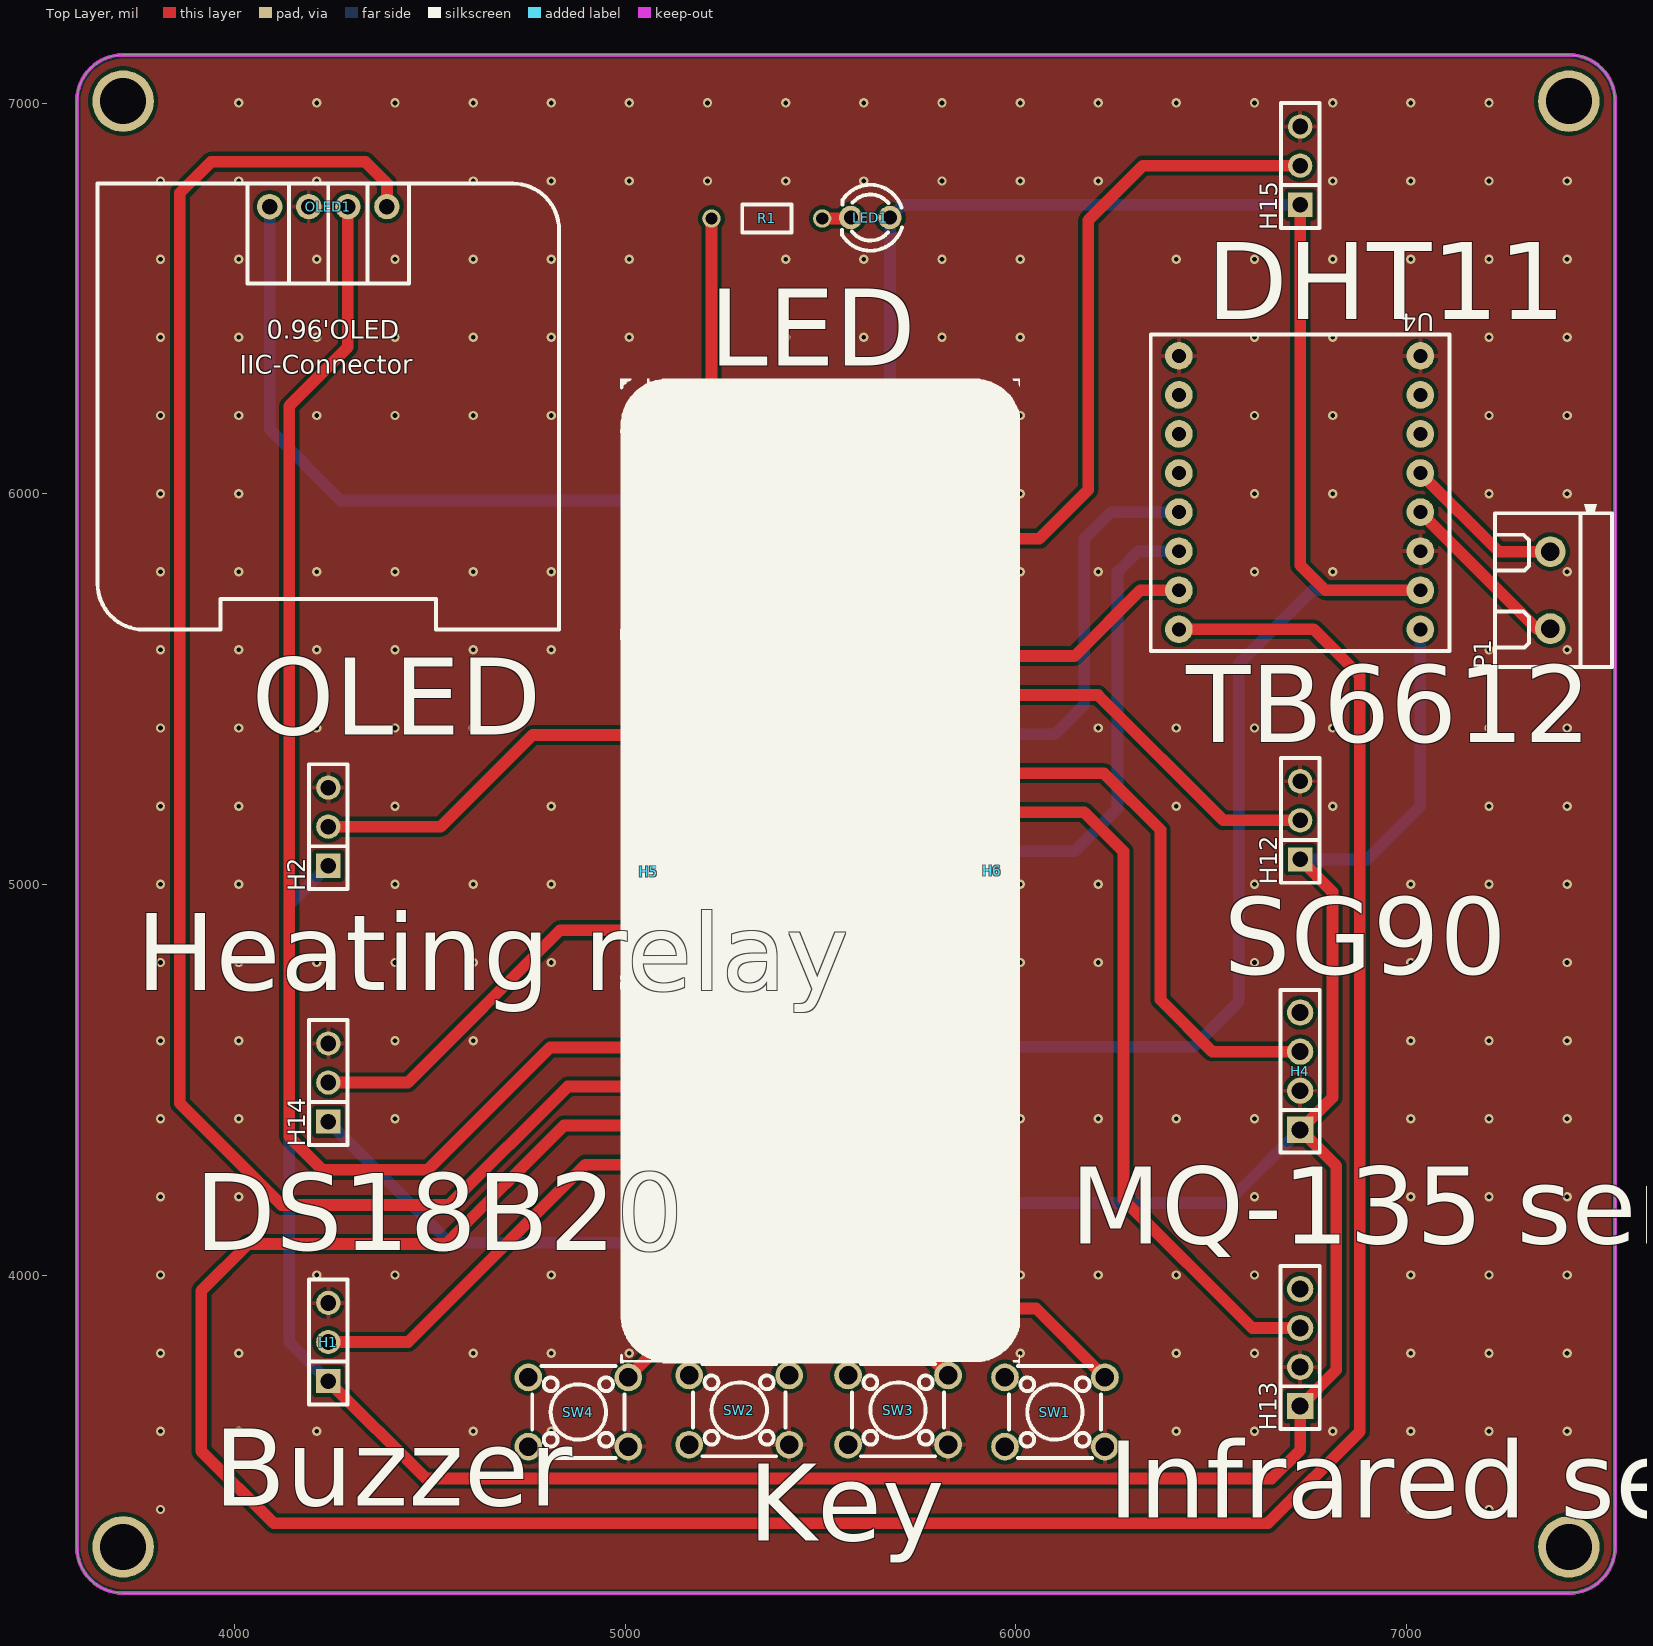
[diagram p0: Top Layer view]
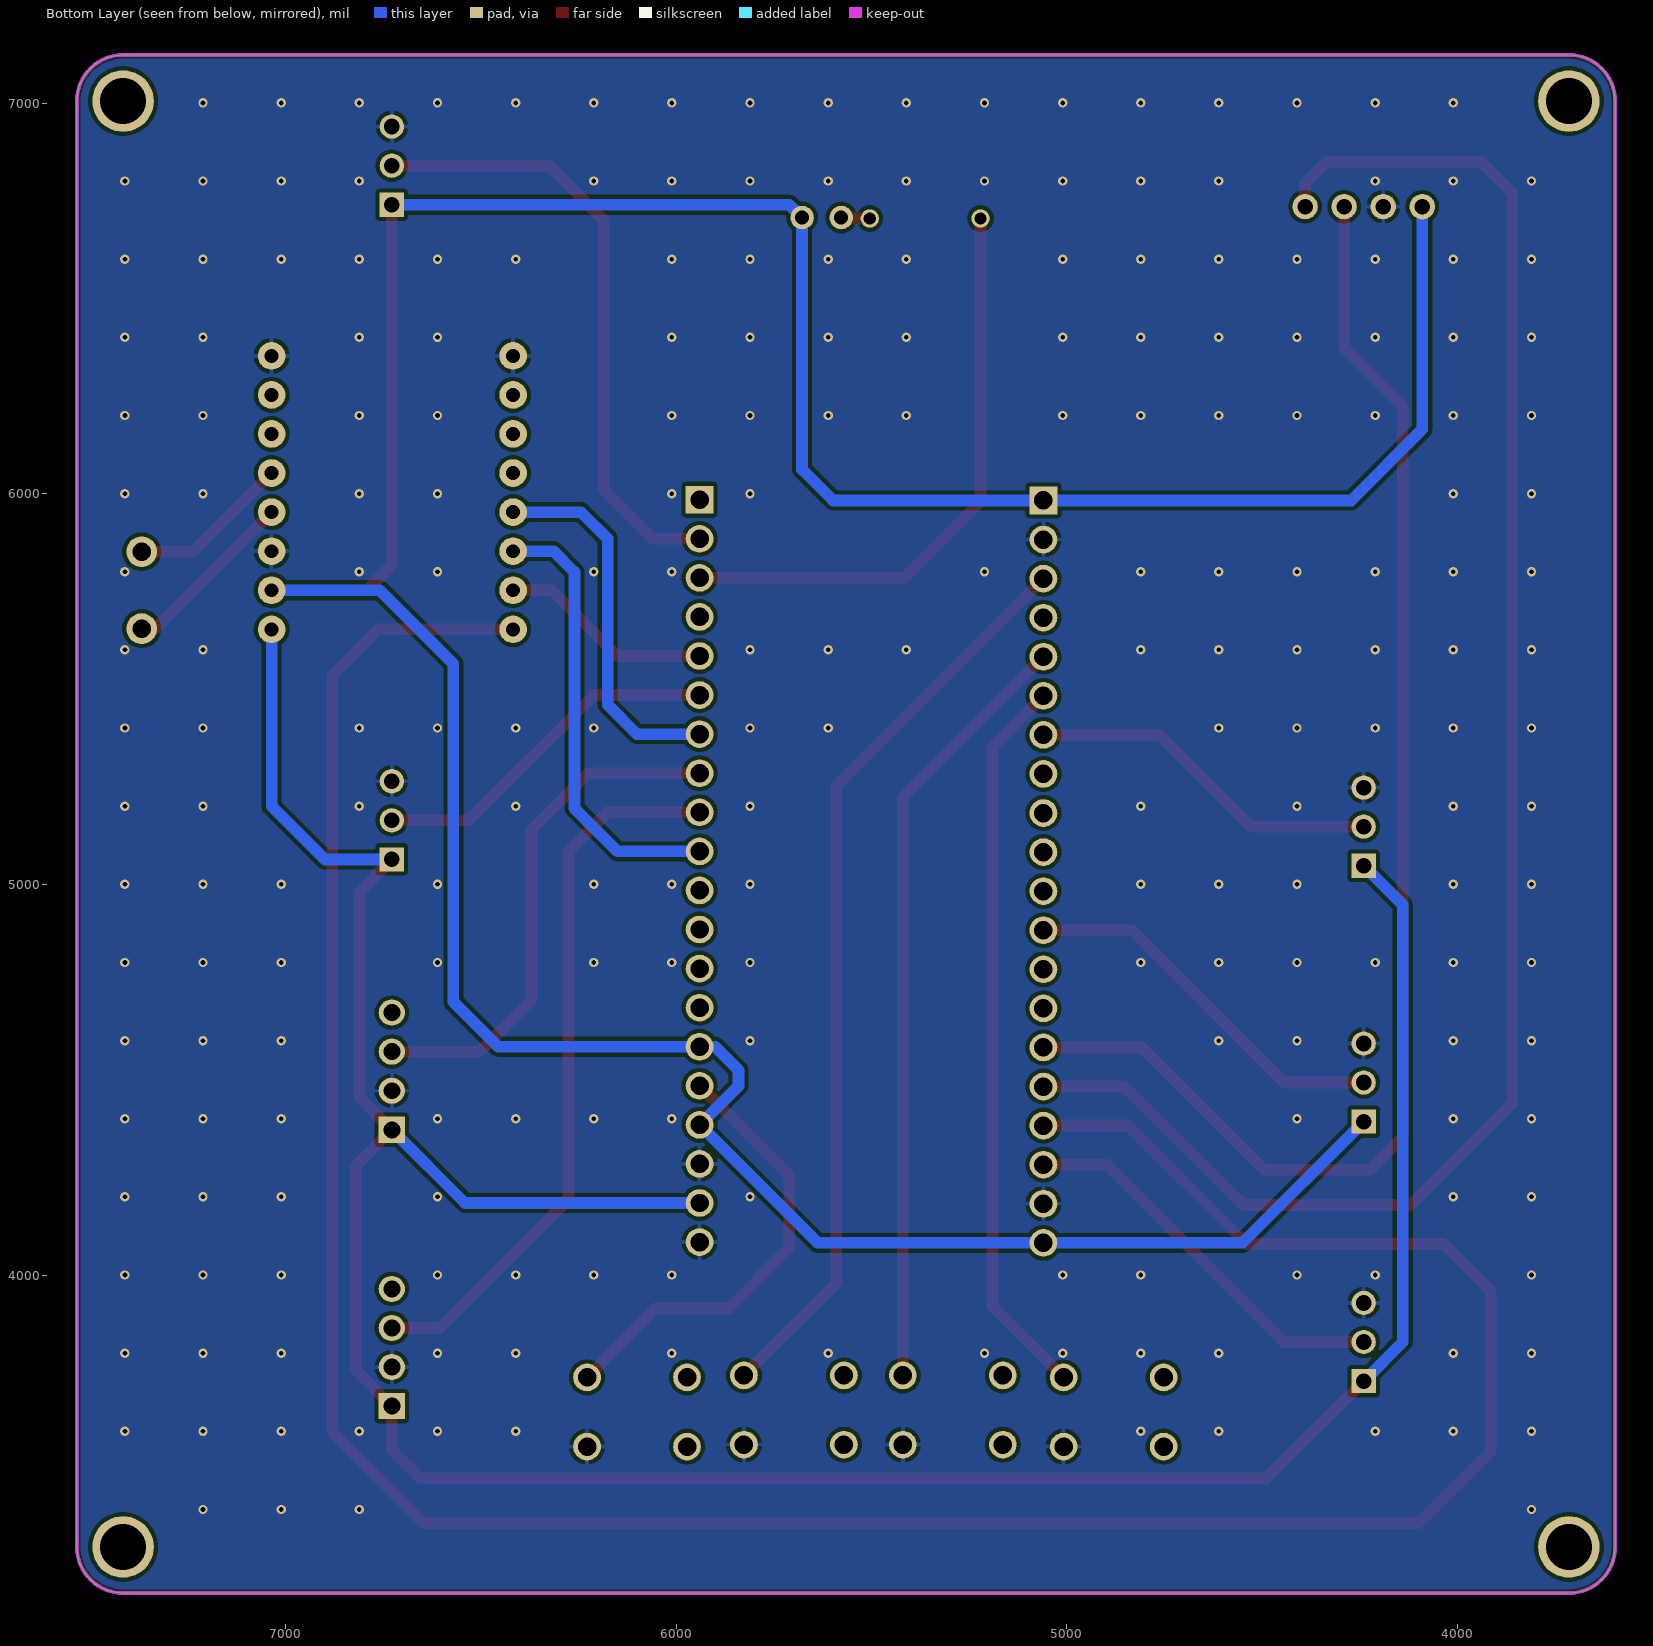
[diagram p1: Bottom Layer view, seen from below]
# Altium PCB MISC49946.pcbdoc
Units mil, origin at the board's own origin, x right, y up, seen from the top; angles counter-clockwise.
Board outline 3937.01 x 3937.01 mil, 2 copper layers (Top Layer, Bottom Layer), stack 62.206 mil thick; 18 components, 37 nets, 109 pads, 223 vias.

## Layer stack, top to bottom
Top Solder Mask Layer: solder mask 0.394, Dk 3.3
Top Layer: signal copper 1.379
Dielectric1: surface 59.449, FR4, Dk 4.5
Bottom Layer: signal copper 1.378
Bottom Solder Mask Layer: solder mask 0.394, Dk 3.3

## Board outline
3714.61,7123.5 ccw(c3714.61,7005.39) 3596.5,7005.39 3596.5,3304.61 ccw(c3714.61,3304.61) 3714.61,3186.5 7415.39,3186.5 ccw(c7415.39,3304.61) 7533.5,3304.61 7533.5,7005.39 ccw(c7415.39,7005.39) 7415.39,7123.5 3714.61,7123.5

## Design rules (kind name [scope] priority, off if disabled: settings)
BoardOutlineClearance copperThickness2oz_1 [All] p2 off: genericclearance=7.99 ignorepadtopadclearanceinfootprint=FALSE except(0: Arc-SplitContinuation Track-SplitContinuation SMDPad-SplitContinuation THPad-SplitContinuation Via-SplitContinuation Fill-SplitContinuation Region-SplitContinuation Poly-SplitContinuation Text-SplitContinuation Hole-SplitContinuation; 5.98: Arc-CutoutEdge Track-CutoutEdge SMDPad-CutoutEdge THPad-CutoutEdge Via-CutoutEdge Text-CutoutEdge; 6.9: Hole-OutlineEdge Hole-CutoutEdge; 10: Poly-OutlineEdge Poly-CutoutEdge; 11.81: Arc-OutlineEdge Track-OutlineEdge SMDPad-OutlineEdge THPad-OutlineEdge Via-OutlineEdge Fill-OutlineEdge Region-OutlineEdge Text-OutlineEdge Fill-CutoutEdge Region-CutoutEdge)
BoardOutlineClearance Plane_innerPlane_1 [All] p4 off: genericclearance=4.02 ignorepadtopadclearanceinfootprint=FALSE except(0: Arc-SplitContinuation Track-SplitContinuation SMDPad-SplitContinuation THPad-SplitContinuation Via-SplitContinuation Fill-SplitContinuation Region-SplitContinuation Poly-SplitContinuation Text-SplitContinuation Hole-SplitContinuation; 5.98: Arc-CutoutEdge Track-CutoutEdge SMDPad-CutoutEdge THPad-CutoutEdge Via-CutoutEdge Text-CutoutEdge; 6.9: Hole-OutlineEdge Hole-CutoutEdge; 10: Poly-OutlineEdge Poly-CutoutEdge; 11.81: Arc-OutlineEdge Track-OutlineEdge SMDPad-OutlineEdge THPad-OutlineEdge Via-OutlineEdge Fill-OutlineEdge Region-OutlineEdge Text-OutlineEdge Fill-CutoutEdge Region-CutoutEdge)
BoardOutlineClearance Copper_copperRegion_1 [All] p6 off: genericclearance=4.02 ignorepadtopadclearanceinfootprint=FALSE except(0: Arc-SplitContinuation Track-SplitContinuation SMDPad-SplitContinuation THPad-SplitContinuation Via-SplitContinuation Fill-SplitContinuation Region-SplitContinuation Poly-SplitContinuation Text-SplitContinuation Hole-SplitContinuation; 5.98: Arc-CutoutEdge Track-CutoutEdge SMDPad-CutoutEdge THPad-CutoutEdge Via-CutoutEdge Text-CutoutEdge; 6.9: Hole-OutlineEdge Hole-CutoutEdge; 10: Poly-OutlineEdge Poly-CutoutEdge; 11.81: Arc-OutlineEdge Track-OutlineEdge SMDPad-OutlineEdge THPad-OutlineEdge Via-OutlineEdge Fill-OutlineEdge Region-OutlineEdge Text-OutlineEdge Fill-CutoutEdge Region-CutoutEdge)
BoardOutlineClearance Copper_copperRegion_copperThickness1oz_1 [All] p8 off: genericclearance=4.02 ignorepadtopadclearanceinfootprint=FALSE except(0: Arc-SplitContinuation Track-SplitContinuation SMDPad-SplitContinuation THPad-SplitContinuation Via-SplitContinuation Fill-SplitContinuation Region-SplitContinuation Poly-SplitContinuation Text-SplitContinuation Hole-SplitContinuation; 5.98: Arc-CutoutEdge Track-CutoutEdge SMDPad-CutoutEdge THPad-CutoutEdge Via-CutoutEdge Text-CutoutEdge; 6.9: Hole-OutlineEdge Hole-CutoutEdge; 10: Poly-OutlineEdge Poly-CutoutEdge; 11.81: Arc-OutlineEdge Track-OutlineEdge SMDPad-OutlineEdge THPad-OutlineEdge Via-OutlineEdge Fill-OutlineEdge Region-OutlineEdge Text-OutlineEdge Fill-CutoutEdge Region-CutoutEdge)
BoardOutlineClearance Copper_copperRegion_Copper_copperRegion_1 [All] p10 off: genericclearance=4.02 ignorepadtopadclearanceinfootprint=FALSE except(0: Arc-SplitContinuation Track-SplitContinuation SMDPad-SplitContinuation THPad-SplitContinuation Via-SplitContinuation Fill-SplitContinuation Region-SplitContinuation Poly-SplitContinuation Text-SplitContinuation Hole-SplitContinuation; 5.98: Arc-CutoutEdge Track-CutoutEdge SMDPad-CutoutEdge THPad-CutoutEdge Via-CutoutEdge Text-CutoutEdge; 6.9: Hole-OutlineEdge Hole-CutoutEdge; 10: Poly-OutlineEdge Poly-CutoutEdge; 11.81: Arc-OutlineEdge Track-OutlineEdge SMDPad-OutlineEdge THPad-OutlineEdge Via-OutlineEdge Fill-OutlineEdge Region-OutlineEdge Text-OutlineEdge Fill-CutoutEdge Region-CutoutEdge)
BoardOutlineClearance copperThickness1oz_1 [All] p12: genericclearance=4.02 ignorepadtopadclearanceinfootprint=FALSE except(0: Arc-SplitContinuation Track-SplitContinuation SMDPad-SplitContinuation THPad-SplitContinuation Via-SplitContinuation Fill-SplitContinuation Region-SplitContinuation Poly-SplitContinuation Text-SplitContinuation Hole-SplitContinuation; 5.98: Arc-CutoutEdge Track-CutoutEdge SMDPad-CutoutEdge THPad-CutoutEdge Via-CutoutEdge Text-CutoutEdge; 6.9: Hole-OutlineEdge Hole-CutoutEdge; 10: Poly-OutlineEdge Poly-CutoutEdge; 11.81: Arc-OutlineEdge Track-OutlineEdge SMDPad-OutlineEdge THPad-OutlineEdge Via-OutlineEdge Fill-OutlineEdge Region-OutlineEdge Text-OutlineEdge Fill-CutoutEdge Region-CutoutEdge)
Clearance copperThickness2oz [All] p1 off: gap=7.99 ignorepadtopadclearanceinfootprint=FALSE except(5.98: SMDPad-Track SMDPad-SMDPad THPad-Track SMDPad-THPad THPad-THPad Track-Via SMDPad-Via THPad-Via Via-Via Fill-SMDPad Region-SMDPad Fill-THPad Region-THPad Fill-Via Region-Via Fill-Fill Fill-Region Region-Region Arc-Track Arc-SMDPad Arc-THPad Arc-Via Fill-Arc Region-Arc Arc-Arc Text-Track SMDPad-Text Text-THPad Text-Via Fill-Text Region-Text Arc-Text Text-Text; 6.9: Hole-Track Hole-SMDPad Hole-THPad Hole-Via Fill-Hole Region-Hole Hole-Arc Hole-Text; 10: Poly-Track Poly-SMDPad Poly-THPad Poly-Via Poly-Fill Poly-Region Poly-Poly Poly-Arc Poly-Text Poly-Hole; 11.81: Fill-Track Region-Track)
Clearance Plane_innerPlane [All] p3 off: gap=4.02 ignorepadtopadclearanceinfootprint=FALSE except(5.98: SMDPad-Track SMDPad-SMDPad THPad-Track SMDPad-THPad THPad-THPad Track-Via SMDPad-Via THPad-Via Via-Via Fill-SMDPad Region-SMDPad Fill-THPad Region-THPad Fill-Via Region-Via Fill-Fill Fill-Region Region-Region Arc-Track Arc-SMDPad Arc-THPad Arc-Via Fill-Arc Region-Arc Arc-Arc Text-Track SMDPad-Text Text-THPad Text-Via Fill-Text Region-Text Arc-Text Text-Text; 6.9: Hole-Track Hole-SMDPad Hole-THPad Hole-Via Fill-Hole Region-Hole Hole-Arc Hole-Text; 10: Poly-Track Poly-SMDPad Poly-THPad Poly-Via Poly-Fill Poly-Region Poly-Poly Poly-Arc Poly-Text Poly-Hole; 11.81: Fill-Track Region-Track)
Clearance Copper_copperRegion [All] p5 off: gap=4.02 ignorepadtopadclearanceinfootprint=FALSE except(5.98: SMDPad-Track SMDPad-SMDPad THPad-Track SMDPad-THPad THPad-THPad Track-Via SMDPad-Via THPad-Via Via-Via Fill-SMDPad Region-SMDPad Fill-THPad Region-THPad Fill-Via Region-Via Fill-Fill Fill-Region Region-Region Arc-Track Arc-SMDPad Arc-THPad Arc-Via Fill-Arc Region-Arc Arc-Arc Text-Track SMDPad-Text Text-THPad Text-Via Fill-Text Region-Text Arc-Text Text-Text; 6.9: Hole-Track Hole-SMDPad Hole-THPad Hole-Via Fill-Hole Region-Hole Hole-Arc Hole-Text; 10: Poly-Track Poly-SMDPad Poly-THPad Poly-Via Poly-Fill Poly-Region Poly-Poly Poly-Arc Poly-Text Poly-Hole; 11.81: Fill-Track Region-Track)
Clearance Copper_copperRegion_copperThickness1oz [All] p7 off: gap=4.02 ignorepadtopadclearanceinfootprint=FALSE except(5.98: SMDPad-Track SMDPad-SMDPad THPad-Track SMDPad-THPad THPad-THPad Track-Via SMDPad-Via THPad-Via Via-Via Fill-SMDPad Region-SMDPad Fill-THPad Region-THPad Fill-Via Region-Via Fill-Fill Fill-Region Region-Region Arc-Track Arc-SMDPad Arc-THPad Arc-Via Fill-Arc Region-Arc Arc-Arc Text-Track SMDPad-Text Text-THPad Text-Via Fill-Text Region-Text Arc-Text Text-Text; 6.9: Hole-Track Hole-SMDPad Hole-THPad Hole-Via Fill-Hole Region-Hole Hole-Arc Hole-Text; 10: Poly-Track Poly-SMDPad Poly-THPad Poly-Via Poly-Fill Poly-Region Poly-Poly Poly-Arc Poly-Text Poly-Hole; 11.81: Fill-Track Region-Track)
Clearance Copper_copperRegion_Copper_copperRegion [All] p9 off: gap=4.02 ignorepadtopadclearanceinfootprint=FALSE except(5.98: SMDPad-Track SMDPad-SMDPad THPad-Track SMDPad-THPad THPad-THPad Track-Via SMDPad-Via THPad-Via Via-Via Fill-SMDPad Region-SMDPad Fill-THPad Region-THPad Fill-Via Region-Via Fill-Fill Fill-Region Region-Region Arc-Track Arc-SMDPad Arc-THPad Arc-Via Fill-Arc Region-Arc Arc-Arc Text-Track SMDPad-Text Text-THPad Text-Via Fill-Text Region-Text Arc-Text Text-Text; 6.9: Hole-Track Hole-SMDPad Hole-THPad Hole-Via Fill-Hole Region-Hole Hole-Arc Hole-Text; 10: Poly-Track Poly-SMDPad Poly-THPad Poly-Via Poly-Fill Poly-Region Poly-Poly Poly-Arc Poly-Text Poly-Hole; 11.81: Fill-Track Region-Track)
Clearance copperThickness1oz [All] p11: gap=4.02 ignorepadtopadclearanceinfootprint=FALSE except(5.98: SMDPad-Track SMDPad-SMDPad THPad-Track SMDPad-THPad THPad-THPad Track-Via SMDPad-Via THPad-Via Via-Via Fill-SMDPad Region-SMDPad Fill-THPad Region-THPad Fill-Via Region-Via Fill-Fill Fill-Region Region-Region Arc-Track Arc-SMDPad Arc-THPad Arc-Via Fill-Arc Region-Arc Arc-Arc Text-Track SMDPad-Text Text-THPad Text-Via Fill-Text Region-Text Arc-Text Text-Text; 6.9: Hole-Track Hole-SMDPad Hole-THPad Hole-Via Fill-Hole Region-Hole Hole-Arc Hole-Text; 10: Poly-Track Poly-SMDPad Poly-THPad Poly-Via Poly-Fill Poly-Region Poly-Poly Poly-Arc Poly-Text Poly-Hole; 11.81: Fill-Track Region-Track)
DiffPairsRouting differentialPair [All] p1: maxlimit=6 minlimit=6 mostfreqgap=6 toplayer_minwidth=5 toplayer_prefwidth=10 toplayer_maxwidth=100 toplayer_mingap=6 toplayer_prefgap=6 toplayer_maxgap=6 bottomlayer_minwidth=5 bottomlayer_prefwidth=10 bottomlayer_maxwidth=100 bottomlayer_mingap=6 bottomlayer_prefgap=6 bottomlayer_maxgap=6 maxuncoupledlength=10
HoleToHoleClearance otherClearance [All] p1: gap=11.81 allowstackedmicrovias=TRUE
Length netLength [All] p1: minlimit=0 maxlimit=0
PasteMaskExpansion pasteMaskExpansion [All] p1: expansion=0
PlaneConnect innerPlane [All] p1: planeconnectstyle=Relief reliefexpansion=20 reliefentries=4 reliefconductorwidth=10 reliefairgap=10
PolygonConnect copperRegion_copperThickness1oz [All] p1 off: connectstyle=Relief reliefconductorwidth=10 reliefentries=4 polygonreliefangle="90 Angle" airgapwidth=10 via.connectstyle=Relief via.reliefconductorwidth=10 via.reliefentries=4 via.polygonreliefangle="90 Angle" via.airgapwidth=10
PolygonConnect copperRegion_Copper_copperRegion [All] p2 off: connectstyle=Relief reliefconductorwidth=10 reliefentries=4 polygonreliefangle="90 Angle" airgapwidth=10 via.connectstyle=Relief via.reliefconductorwidth=10 via.reliefentries=4 via.polygonreliefangle="90 Angle" via.airgapwidth=10
PolygonConnect copperRegion [All] p3: connectstyle=Relief reliefconductorwidth=10 reliefentries=4 polygonreliefangle="90 Angle" airgapwidth=10 via.connectstyle=Relief via.reliefconductorwidth=10 via.reliefentries=4 via.polygonreliefangle="90 Angle" via.airgapwidth=10
RoutingVias viaSize [All] p1: holewidth=12.01 width=24.02 viastyle="Through Hole" minholewidth=11.81 minwidth=19.68 maxholewidth=248.03 maxwidth=393.7
SolderMaskExpansion solderMaskExpansion [IsVia] p1: expansion=-1000 istentingtop=TRUE
SolderMaskExpansion solderMaskExpansion [All] p2: expansion=2 istentingtop=FALSE
Width copperThickness2oz_2 [All] p1 off: maxlimit=100 minlimit=8 preferedwidth=10
Width copperThickness1oz_2 [All] p2: maxlimit=100 minlimit=5 preferedwidth=10

## Components (designator, comment, footprint, x,y, rotation, side; value= is the part's Value field where it differs from the comment)
H1 "" HDR-TH_3P-P2.54-V-F 4240,3829.14 r90 top
H2 "" HDR-TH_3P-P2.54-V-F 4240,5148.1 r90 top
H4 "" HDR-TH_4P-P2.54-V-F 6727.5,4522.29 r90 top
H5 "" HDR-TH_20P-P2.54-V-F 5059.74,5033.05 r270 top
H6 "" HDR-TH_20P-P2.54-V-F 5939.74,5034.94 r270 top
H12 "" HDR-TH_3P-P2.54-V-F 6727.5,5164.4 r90 top
H13 "" HDR-TH_4P-P2.54-V-F 6727.5,3815.05 r90 top
H14 "" HDR-TH_3P-P2.54-V-F 4240,4493.24 r90 top
H15 "" HDR-TH_3P-P2.54-V-F 6727.5,6840 r90 top
LED1 "" LED_TH-3mm 5627.35,6707.23 r180 top
OLED1 "" 0.96OLED_4P 4240,6735 r0 top
P1 "KF301-2P terminal block" CONN-TH_XY301V-A-5.0-2P 7367.76,5753.51 r90 top
R1 "220Ω" Res_1/8W 5362.36,6707.23 r180 top
SW1 "" SW-TH_4P-L6.0-W6.0-P4.50-LS6.5 6099.85,3650 r180 top
SW2 "" SW-TH_4P-L6.0-W6.0-P4.50-LS6.5 5291.62,3655 r180 top
SW3 "" SW-TH_4P-L6.0-W6.0-P4.50-LS6.5 5698.23,3655 r180 top
SW4 "" SW-TH_4P-L6.0-W6.0-P4.50-LS6.5 4880,3650 r180 top
U4 "" tb6612 7035,5653.24 r180 top

## Footprints (in the part's own frame and the unit in brackets; to place one, negate y for a bottom-side part, rotate by r counter-clockwise, add the part's x,y. Pads: shape width x height; smd on the part's side, far side on the other; paste and mask are expansions set on the pad)
0.96OLED_4P [mm]
  round 1.65 hole 1 copper offset 0,0: 1(-3.81,-0.001) 2(-1.27,0.002) 3(1.27,0.002) 4(3.81,0.002)
  silkscreen extent -15,-27.5 15,1.5
CONN-TH_XY301V-A-5.0-2P [mm]
  round 2 hole 1.2: 1(-2.5,0) 2(2.5,0)
  silkscreen extent -5,-4 5.6,3.6
HDR-TH_3P-P2.54-V-F [mil]
  rect 62x62 hole 40.16: 1(-100,0)
  round 62 hole 40.16: 2(0,0) 3(100,0)
  silkscreen extent -160,-49 160,49
HDR-TH_4P-P2.54-V-F [mm]
  rect 1.7x1.7 hole 1.1: 1(-3.81,0)
  round 1.7 hole 1.1: 2(-1.27,0) 3(1.27,0) 4(3.81,0)
  silkscreen extent -5.29,-1.27 5.29,1.27
HDR-TH_20P-P2.54-V-F [mm]
  rect 1.8x1.8 hole 1.2: 1(-24.13,0)
  round 1.8 hole 1.2: 2(-21.59,0) 3(-19.05,0) 4(-16.51,0) 5(-13.97,0) 6(-11.43,0) 7(-8.89,0) 8(-6.35,0) 9(-3.81,0) 10(-1.27,0) 11(1.27,0) 12(3.81,0) 13(6.35,0) 14(8.89,0) 15(11.43,0) 16(13.97,0) 17(16.51,0) 18(19.05,0) 19(21.59,0) 20(24.13,0)
  silkscreen extent -25.65,-1.25 25.65,1.25
LED_TH-3mm [mil]
  round 60 hole 36 paste+0 mask+2: 1(-50,0) 2(50,0)
  silkscreen extent -81,-84 72,85
Res_1/8W [mil]
  round 47.2 hole 31.5 paste+0 mask+2: 1(-141.7,2.48) 2(141.7,2.48)
  silkscreen extent -63,-33 63,38
SW-TH_4P-L6.0-W6.0-P4.50-LS6.5 [mm]
  round 1.8 hole 1.2: 1(-3.25,2.25) 2(3.25,2.25) 3(-3.25,-2.25) 4(3.25,-2.25)
  silkscreen extent -3,-3 3,3
tb6612 [mm]
  round 1.8 hole 0.9: 1(0,0) 2(0,-2.54) 3(0,-5.08) 4(0,-7.62) 5(0,-10.16) 6(0,-12.7) 7(0,-15.24) 8(0,-17.78) 9(15.697,-17.78) 10(15.697,-15.24) 11(15.697,-12.7) 12(15.697,-10.16) 13(15.697,-7.62) 14(15.697,-5.08) 15(15.697,-2.54) 16(15.697,0)
  silkscreen extent -1.91,-19.18 17.53,1.4

## Free pads (board coordinates)
  round 157.48 hole 118.11: 1(3714.61,7005.39) 1(3714.61,3304.61) 1(7415.39,7005.39) 1(7415.39,3304.61)

## Via types
v1: diameter 24.02, hole 12, Top Layer to Bottom Layer, 223 vias

## Nets (pads, with @x,y where several pads share a name; then routed paths per layer and width w, separated by ;. In a path a pad name is that pad's centre, name@x,y a point inside that pad or via, vN(x,y) a via of type N, cw(c..) or ccw(c..) an arc to the next point about the centre after c; other vN are vias at no path point)
$1N17195: LED1.2 R1.1 | length 74.3
  Top Layer w30: R1.1 5574.87,6704.75 LED1.2
$1N17231: P1.1 U4.4 | length 456.3
  Top Layer w30: U4.4 7333.15,5655.09 P1.1
$1N17232: P1.2 U4.5 | length 416.1
  Top Layer w30: U4.5 7236.3,5851.94 P1.2
+5V: H1.1 H2.1 H4.1 H6.19 H12.1 H13.1 U4.1 | length 7361.7
  Top Layer w30: H1.1 4489.14,3480 6655,3480 6727.5,3552.5 H13.1 6820,3757.55 6820,4279.79 H4.1 6810,4454.79 6810,4981.9 H12.1
  Bottom Layer w30: H1.1 4140,3829.14 4140,4948.1 H2.1 ; H6.19 6540.15,4184.94 H4.1 ; H12.1 6899.4,5064.4 7035,5200 U4.1
A0: H6.14
A1: H6.13
A2: H6.12
A3: H6.11
A4: H6.10 U4.14 | length 1149.9
  Bottom Layer w30: H6.10 6149.94,5084.94 6260,5195 6260,5800 6313.24,5853.24 U4.14
A5: H6.9 H13.3 | length 1855.8
  Top Layer w30: H6.9 6175.06,5184.94 6275,5085 6275,4195 6604.95,3865.05 H13.3
A6: H4.3 H6.8 | length 1337.8
  Top Layer w30: H6.8 6225.06,5284.94 6370,5140 6370,4705 6502.71,4572.29 H4.3
A7: H6.7 U4.13 | length 961.6
  Bottom Layer w30: H6.7 6099.94,5384.94 6175,5460 6175,5885 6243.24,5953.24 U4.13
A8: H2.2 H5.7 | length 917.1
  Top Layer w30: H2.2 4528.1,5148.1 4763.05,5383.05 H5.7
A9: H5.5 SW2.3 | length 1988.5
  Top Layer w30: H5.5 5419.57,5223.22 SW2.3
A10: H5.6 SW4.3 | length 1873.8
  Top Layer w30: SW4.3 5190,3920.63 5190,5352.79 H5.6
A11: H5.3 SW3.3 | length 2356.9
  Top Layer w30: H5.3 5590,5252.79 5590,3979.76 SW3.3
A12: H5.4
A15: H5.11
B0: H6.6 H12.2 | length 920.5
  Top Layer w30: H6.6 6210.06,5484.94 6530.6,5164.4 H12.2
B1: H6.5 U4.15 | length 547
  Top Layer w30: H6.5 6149.94,5584.94 6318.24,5753.24 U4.15
B3: H5.12 H14.2 | length 981.2
  Top Layer w30: H14.2 4443.24,4493.24 4833.05,4883.05 H5.12
B4: H5.13
B5: H5.14
B6: H5.15 OLED1.3 | length 3526.8
  Top Layer w30: OLED1.3@4290,6735.05 4290,6375 4140,6225 4140,4355 4225,4270 4495,4270 4808.05,4583.05 H5.15
B7: H5.16 OLED1.4 | length 4408.8
  Top Layer w30: OLED1.4@4390,6735.05 4390,6795 4335,6850 3940,6850 3860,6770 3860,4440 4120,4180 4550,4180 4853.05,4483.05 H5.16
B8: H5.17 U4.16 | length 7315.9
  Top Layer w30: H5.17 4843.05,4383.05 4540,4080 4035,4080 3915,3960 3915,3550 4100,3365 6645,3365 6880,3600 6880,5535 6761.76,5653.24 U4.16
B9: H1.2 H5.18 | length 1007.8
  Top Layer w30: H1.2 4444.14,3829.14 4898.05,4283.05 H5.18
B10: H6.4
B11: H6.3 R1.2 | length 1525
  Top Layer w30: R1.2 5220.66,5979.34 5415.06,5784.94 H6.3
B12: H6.2 H15.2 | length 1587.6
  Top Layer w30: H6.2 6059.94,5884.94 6185,6010 6185,6700 6325,6840 H15.2
B13: H5.10
B14: H5.9
B15: H5.8
C13: H6.16 SW1.3 | length 1165.2
  Top Layer w30: H6.16 5710,4255.2 5710,4070 5865,3915 6051.38,3915 SW1.3
GND: H1.3 H2.3 H4.2 H5.2 H5.19 H6.18 H6.20 H12.3 H13.2 H14.3 H15.3 OLED1.2 SW1.1 SW2.1 SW3.1 SW4.1 U4.3 U4.8 U4.9
  other v1: 3810.6,3400.6 6810.6,3400.6 7010.6,3400.6 7210.6,3400.6 3810.6,3600.6 4010.6,3600.6 4210.6,3600.6 4610.6,3600.6 4810.6,3600.6 6410.6,3600.6 6610.6,3600.6 6810.6,3600.6 7010.6,3600.6 7210.6,3600.6 7410.6,3600.6 3810.6,3800.6 4010.6,3800.6 4610.6,3800.6 4810.6,3800.6 5010.6,3800.6 5210.6,3800.6 5610.6,3800.6 6010.6,3800.6 6410.6,3800.6 6610.6,3800.6 7010.6,3800.6 7210.6,3800.6 7410.6,3800.6 3810.6,4000.6 4210.6,4000.6 4410.6,4000.6 4810.6,4000.6 5010.6,4000.6 6010.6,4000.6 6210.6,4000.6 6410.6,4000.6 6610.6,4000.6 7010.6,4000.6 7210.6,4000.6 7410.6,4000.6 3810.6,4200.6 4010.6,4200.6 5810.6,4200.6 6610.6,4200.6 7010.6,4200.6 7210.6,4200.6 7410.6,4200.6 3810.6,4400.6 4010.6,4400.6 4410.6,4400.6 6010.6,4400.6 6210.6,4400.6 6410.6,4400.6 6610.6,4400.6 7010.6,4400.6 7210.6,4400.6 7410.6,4400.6 3810.6,4600.6 4010.6,4600.6 4410.6,4600.6 4610.6,4600.6 5810.6,4600.6 7010.6,4600.6 7210.6,4600.6 7410.6,4600.6 3810.6,4800.6 4010.6,4800.6 4210.6,4800.6 4410.6,4800.6 4610.6,4800.6 4810.6,4800.6 5810.6,4800.6 6010.6,4800.6 6210.6,4800.6 6610.6,4800.6 7010.6,4800.6 7210.6,4800.6 7410.6,4800.6 3810.6,5000.6 4010.6,5000.6 4410.6,5000.6 4610.6,5000.6 4810.6,5000.6 5810.6,5000.6 6010.6,5000.6 6210.6,5000.6 6610.6,5000.6 7010.6,5000.6 7210.6,5000.6 7410.6,5000.6 3810.6,5200.6 4010.6,5200.6 4410.6,5200.6 4810.6,5200.6 5810.6,5200.6 6410.6,5200.6 6810.6,5200.6 7210.6,5200.6 7410.6,5200.6 3810.6,5400.6 4010.6,5400.6 4210.6,5400.6 4410.6,5400.6 4610.6,5400.6 5610.6,5400.6 5810.6,5400.6 6210.6,5400.6 6410.6,5400.6 6610.6,5400.6 6810.6,5400.6 7210.6,5400.6 7410.6,5400.6 3810.6,5600.6 4010.6,5600.6 4210.6,5600.6 4410.6,5600.6 4610.6,5600.6 4810.6,5600.6 5410.6,5600.6 5610.6,5600.6 5810.6,5600.6 7210.6,5600.6 7410.6,5600.6 3810.6,5800.6 4010.6,5800.6 4210.6,5800.6 4410.6,5800.6 4610.6,5800.6 4810.6,5800.6 5210.6,5800.6 6010.6,5800.6 6210.6,5800.6 6610.6,5800.6 6810.6,5800.6 7410.6,5800.6 3810.6,6000.6 4010.6,6000.6 5810.6,6000.6 6010.6,6000.6 6610.6,6000.6 6810.6,6000.6 7210.6,6000.6 7410.6,6000.6 3810.6,6200.6 4010.6,6200.6 4210.6,6200.6 4410.6,6200.6 4610.6,6200.6 4810.6,6200.6 5010.6,6200.6 5410.6,6200.6 5610.6,6200.6 5810.6,6200.6 6010.6,6200.6 6610.6,6200.6 6810.6,6200.6 7210.6,6200.6 7410.6,6200.6 3810.6,6400.6 4010.6,6400.6 4210.6,6400.6 4410.6,6400.6 4610.6,6400.6 4810.6,6400.6 5010.6,6400.6 5410.6,6400.6 5610.6,6400.6 5810.6,6400.6 6010.6,6400.6 6610.6,6400.6 6810.6,6400.6 7210.6,6400.6 7410.6,6400.6 3810.6,6600.6 4010.6,6600.6 4210.6,6600.6 4410.6,6600.6 4610.6,6600.6 4810.6,6600.6 5010.6,6600.6 5410.6,6600.6 5610.6,6600.6 5810.6,6600.6 6010.6,6600.6 6410.6,6600.6 6610.6,6600.6 6810.6,6600.6 7010.6,6600.6 7210.6,6600.6 7410.6,6600.6 3810.6,6800.6 4010.6,6800.6 4210.6,6800.6 4610.6,6800.6 4810.6,6800.6 5010.6,6800.6 5210.6,6800.6 5410.6,6800.6 5610.6,6800.6 5810.6,6800.6 6010.6,6800.6 6210.6,6800.6 6810.6,6800.6 7010.6,6800.6 7210.6,6800.6 7410.6,6800.6 4010.6,7000.6 4210.6,7000.6 4410.6,7000.6 4610.6,7000.6 4810.6,7000.6 5010.6,7000.6 5210.6,7000.6 5410.6,7000.6 5610.6,7000.6 5810.6,7000.6 6010.6,7000.6 6210.6,7000.6 6410.6,7000.6 6610.6,7000.6 6810.6,7000.6 7010.6,7000.6 7210.6,7000.6
VBAT: H6.1
VCC: H5.1 H5.20 H6.15 H6.17 H14.1 H15.1 LED1.1 OLED1.1 U4.2 | length 9575.8
  Top Layer w30: H15.1 6727.5,5817.5 6791.76,5753.24 U4.2
  Bottom Layer w30: OLED1.1 4090,6165 4271.95,5983.05 H5.1 5598.05,5983.05 5677.35,6062.35 LED1.1 5710.12,6740 H15.1 ; H14.1 4550.19,4083.05 H5.20 5637.85,4083.05 H6.17 5840,4484.68 5840,4525 5899.94,4584.94 H6.15 6454.94,4584.94 6570,4700 6570,5565 6758.24,5753.24 U4.2
pads on no net: H4.4 H13.4 SW1.2 SW1.4 SW2.2 SW2.4 SW3.2 SW3.4 SW4.2 SW4.4 U4.6 U4.7 U4.10 U4.11 U4.12

## Polygon pours and split planes (outlines as drawn)
GND on Bottom Layer (solid, remove dead copper, pour order 2): 3525,7245 3525,3080 7700,3080 7700,7245
GND on Top Layer (solid, remove dead copper, pour order 2): 3000,7415 3000,3000 7930,3000 7930,7415

## Keep-outs
Board Outline Layer:
  the board outline again, w10

## Silkscreen, mask and mechanical layers (free items; w line width, h text height)
Top Silkscreen Layer:
  drawing of 450 lines, arcs and shapes, not listed
  text "DHT11" at 6488.89,6446.82 h196.85
  text "LED" at 5215.32,6327.95 h196.85
  text "OLED" at 4043.44,5383.51 h196.85
  text "TB6612" at 6435.8,5364.61 h196.85
  text "SG90" at 6531.54,4770.92 h196.85
  text "Heating relay" at 3747.98,4729.25 h196.85
  text "MQ-135 sensor" at 6139.33,4080.38 h196.85
  text "DS18B20" at 3898.04,4064.56 h196.85
  text "Buzzer" at 3946.81,3410 h196.85
  text "Infrared sensor" at 6235.97,3380 h196.85
  text "Key" at 5315,3320 h196.85